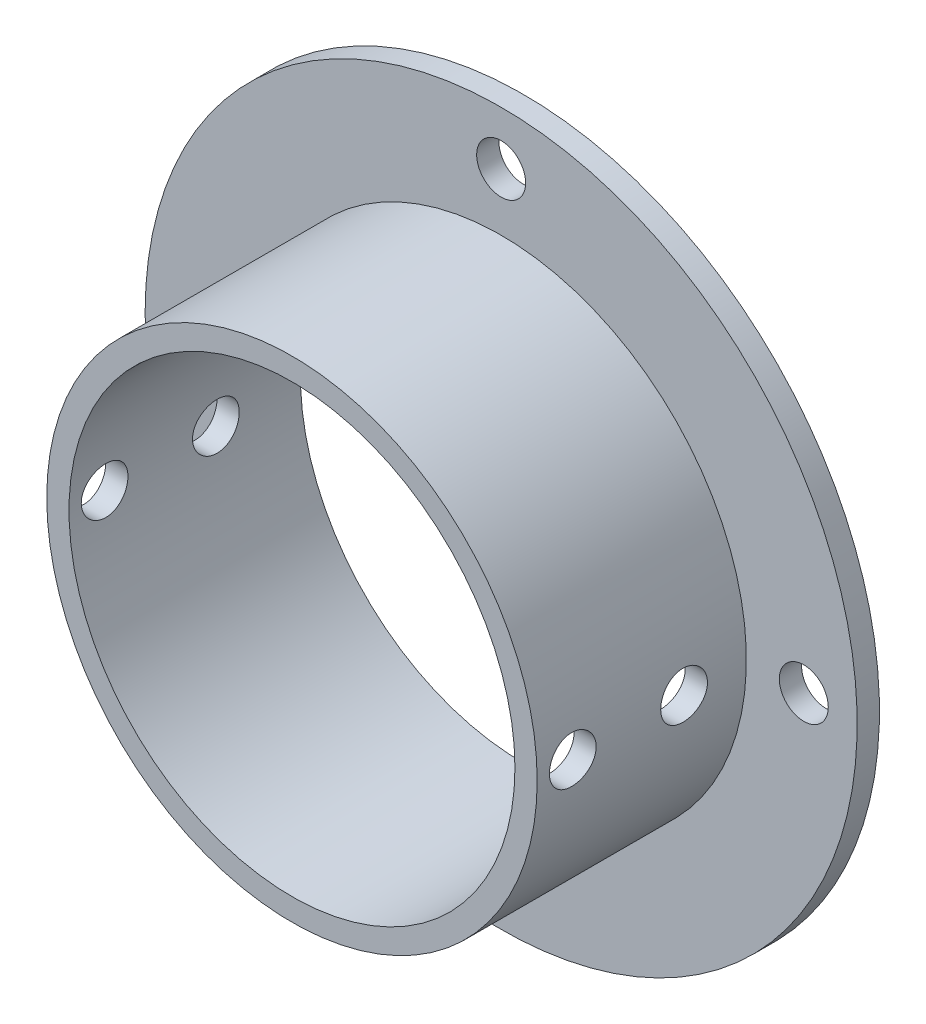
from build123d import *

# Parameters (mm, degrees)
SKETCH_1_R               = 55.1
SKETCH_1_R_2             = 50.1
EXTRUDE_1_DEPTH          = 52
SKETCH_2_R               = 80
EXTRUDE_2_DEPTH          = 5
SKETCH_3_R               = 5.5
CUT_EXTRUDE_1_DEPTH      = 14
PATTERN_CIRCULAR_1_COUNT = 4
CUT_EXTRUDE_START        = -66
SKETCH_4_R               = 50.1
CUT_EXTRUDE_2_DEPTH      = 66
SKETCH_6_R               = 5.25
CUT_EXTRUDE_3_DEPTH      = 103


with BuildPart() as part:
    # 草图1 → 凸台-拉伸1 (new body)
    with BuildSketch(Plane.XY):
        with Locations(Location((0, 0, 0), (0, 0, 180))):
            Circle(SKETCH_1_R)
        with Locations(Location((0, 0, 0), (0, 0, 180))):
            Circle(SKETCH_1_R_2, mode=Mode.SUBTRACT)
    extrude(amount=EXTRUDE_1_DEPTH)

    # 草图2 → 凸台-拉伸2 (add)
    with BuildSketch(Plane(origin=(0, 0, 0), x_dir=(-1, 0, 0), z_dir=(0, 0, -1))):
        Circle(SKETCH_2_R)
    extrude(amount=-EXTRUDE_2_DEPTH)

    # 草图3 → 切除-拉伸1 (cut)
    with BuildSketch(Plane.XY.offset(5)):
        with Locations((0, 68)):
            Circle(SKETCH_3_R)
    cut_extrude_1 = extrude(amount=-CUT_EXTRUDE_1_DEPTH, mode=Mode.SUBTRACT)

    # 阵列(圆周)1: 切除-拉伸1 ×4 about axis
    pattern_circular_1_axis = Axis((0, 0, 0), (0, 0, 1))
    for i in range(1, PATTERN_CIRCULAR_1_COUNT):
        add(cut_extrude_1.rotate(pattern_circular_1_axis, i * 360 / PATTERN_CIRCULAR_1_COUNT), mode=Mode.SUBTRACT)

    # 草图4 → 切除-拉伸2 (cut)
    with BuildSketch(Plane.XY.offset(5).offset(CUT_EXTRUDE_START)):
        with Locations(Location((0, 0, 0), (0, 0, 180))):
            Circle(SKETCH_4_R)
    extrude(amount=CUT_EXTRUDE_2_DEPTH, mode=Mode.SUBTRACT)

    # 草图6 → 切除-拉伸3 (cut, symmetric)
    with BuildSketch(Plane(origin=(0, 0, 0), x_dir=(0, -1, 0), z_dir=(1, 0, 0))):
        with Locations(Location((0, -19, 0), (0, 0, 90))):
            Circle(SKETCH_6_R)
        with Locations(Location((0, -44, 0), (0, 0, 90))):
            Circle(SKETCH_6_R)
    extrude(amount=CUT_EXTRUDE_3_DEPTH, both=True, mode=Mode.SUBTRACT)


solid = part.part
